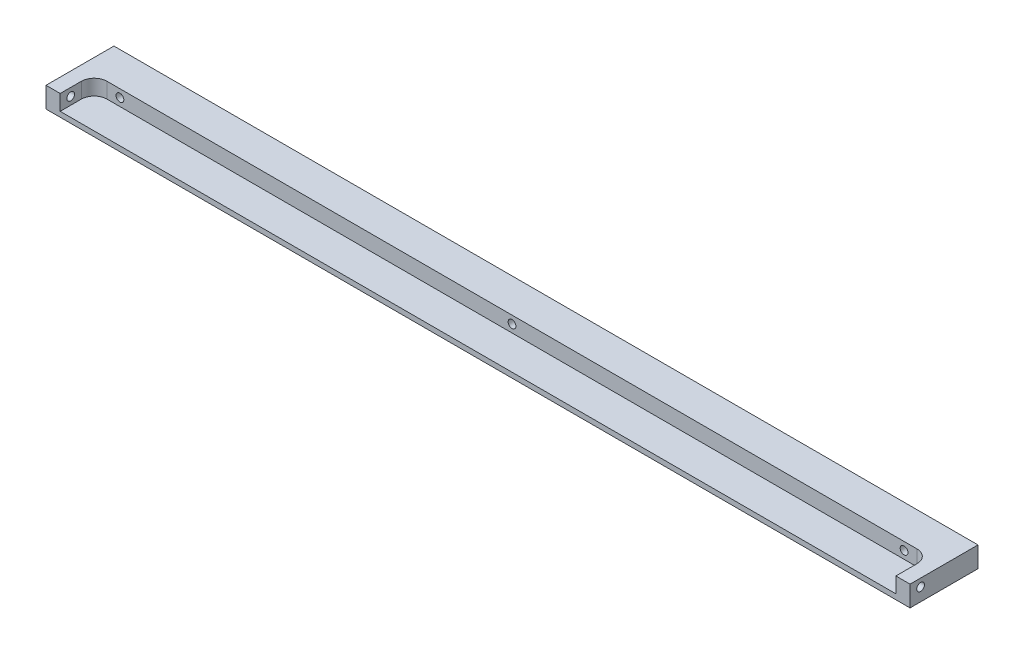
from build123d import *

# Parameters (mm, degrees)
SKETCH1_W                 = 670
SKETCH1_H                 = 52.68545994
BOSS_EXTRUDE1_DEPTH       = 16
SKETCH3_W                 = 648
SKETCH3_H                 = 81.022530329
CUT_EXTRUDE2_DEPTH        = 12
FILLET1_R                 = 10
F_6_0MM_DOWEL_HOLE1_D     = 6
F_6_0MM_DOWEL_HOLE1_DEPTH = 11
F_6_0MM_DOWEL_HOLE2_D     = 6


with BuildPart() as part:
    # Sketch1 → Boss-Extrude1 (new body)
    with BuildSketch(Plane(origin=(0, 0, 0), x_dir=(1, 0, 0), z_dir=(0, 1, 0))):
        Rectangle(SKETCH1_W, SKETCH1_H)
    extrude(amount=BOSS_EXTRUDE1_DEPTH)

    # Sketch3 → Cut-Extrude2 (cut)
    with BuildSketch(Plane(origin=(0, 16, 0), x_dir=(1, 0, 0), z_dir=(0, 1, 0))):
        with Locations((0, -40.511265165)):
            Rectangle(SKETCH3_W, SKETCH3_H)
    extrude(amount=-CUT_EXTRUDE2_DEPTH, mode=Mode.SUBTRACT)

    # Fillet1
    fillet1_edges = [part.edges().sort_by_distance(p)[0] for p in [
        (324, 10, 0),
        (-324, 10, 0),
    ]]
    fillet(fillet1_edges, radius=FILLET1_R)

    # Ø6.0mm Dowel Hole1
    with Locations(Plane.ZY.offset(-324)):
        with Locations((18.171364985, 10)):
            f_6_0mm_dowel_hole1 = Hole(F_6_0MM_DOWEL_HOLE1_D / 2, depth=F_6_0MM_DOWEL_HOLE1_DEPTH)

    # Mirror1: Ø6.0mm Dowel Hole1 across plane
    add(f_6_0mm_dowel_hole1.mirror(Plane(origin=(0, 0, 0), x_dir=(0, 0, 1), z_dir=(1, 0, 0))), mode=Mode.SUBTRACT)

    # Ø6.0mm Dowel Hole2 (through all)
    with Locations(Plane.XY):
        with Locations((304, 10), (0, 10)):
            f_6_0mm_dowel_hole2 = Hole(F_6_0MM_DOWEL_HOLE2_D / 2)

    # Mirror2: Ø6.0mm Dowel Hole2 across plane
    add(f_6_0mm_dowel_hole2.mirror(Plane(origin=(0, 0, 0), x_dir=(0, 0, 1), z_dir=(1, 0, 0))), mode=Mode.SUBTRACT)


solid = part.part
